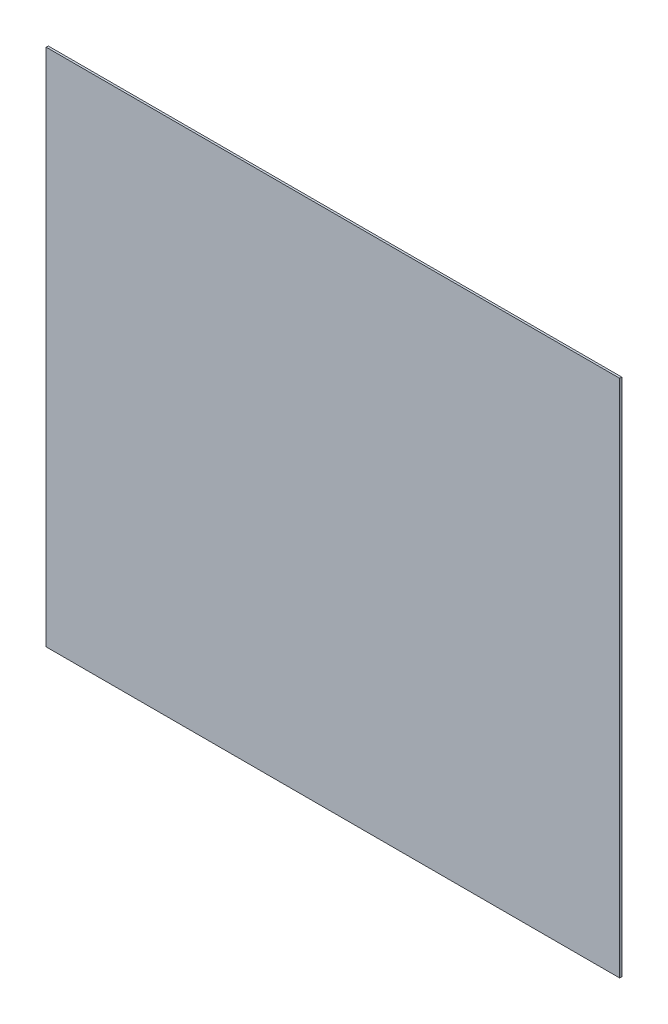
from build123d import *

# Parameters (mm, degrees)
SKETCH_1_W      = 817.222167284
SKETCH_1_H      = 740.222167284
EXTRUDE_1_DEPTH = 3


with BuildPart() as part:
    # 草图1 → 凸台-拉伸1 (new body)
    with BuildSketch(Plane.XY):
        Rectangle(SKETCH_1_W, SKETCH_1_H)
    extrude(amount=EXTRUDE_1_DEPTH)


solid = part.part
